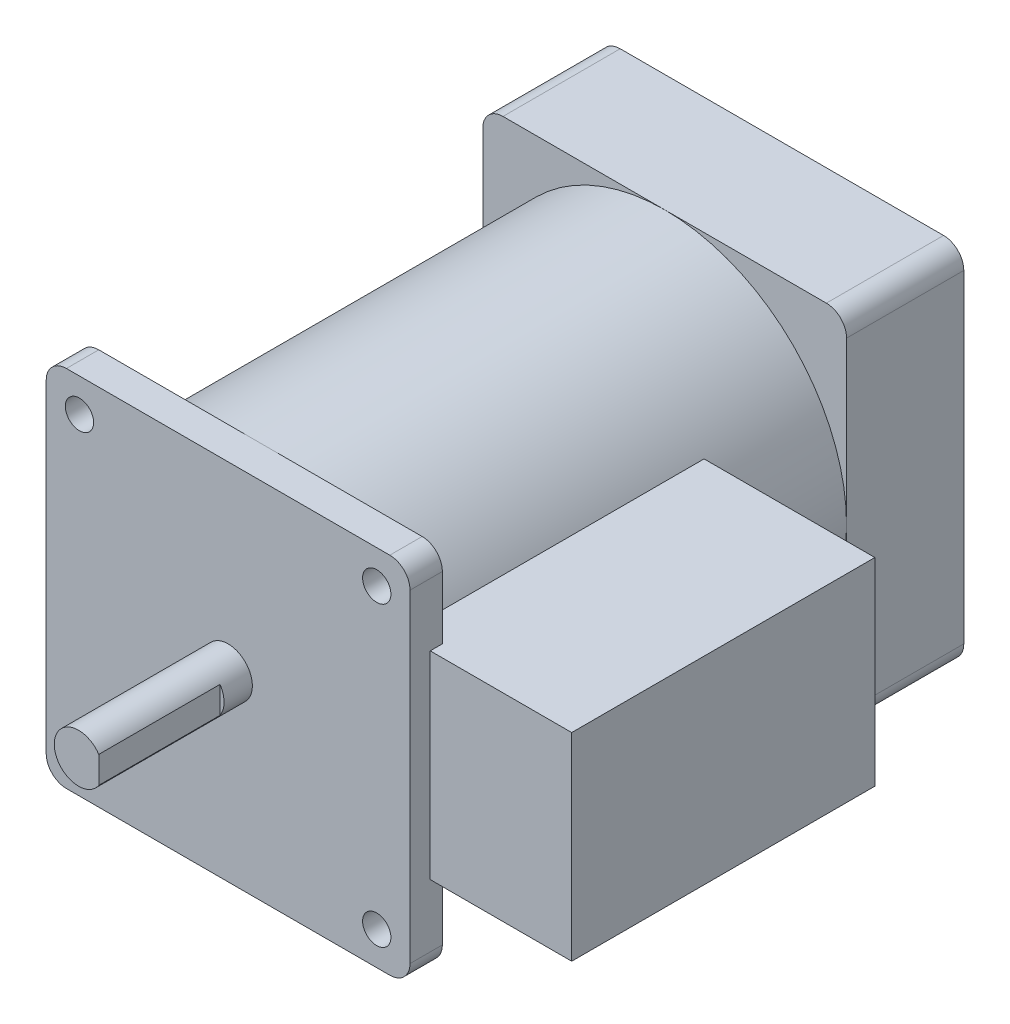
from build123d import *

# Parameters (mm, degrees)
SKETCH_1_W               = 90
SKETCH_1_H               = 90
EXTRUDE_1_DEPTH          = 8
SKETCH_2_R               = 45
EXTRUDE_2_DEPTH          = 100
SKETCH_3_W               = 90
SKETCH_3_H               = 90
EXTRUDE_3_DEPTH          = 29
SKETCH_4_R               = 6
EXTRUDE_4_DEPTH          = 37
SKETCH_6_W               = 75
SKETCH_6_H               = 49
EXTRUDE_5_DEPTH          = 80
SKETCH_7_R               = 3.5
CUT_EXTRUDE_1_DEPTH      = 8
FILLET_1_R               = 5
FILLET_2_R               = 5
SKETCH_9_W               = 30
SKETCH_9_H               = 15.937749453
CUT_EXTRUDE_2_DEPTH      = 1
PATTERN_CIRCULAR_1_COUNT = 4


with BuildPart() as part:
    # 草图1 → 凸台-拉伸1 (new body)
    with BuildSketch(Plane.XY):
        Rectangle(SKETCH_1_W, SKETCH_1_H)
    extrude(amount=EXTRUDE_1_DEPTH)

    # 草图2 → 凸台-拉伸2 (add)
    with BuildSketch(Plane(origin=(0, 0, 0), x_dir=(-1, 0, 0), z_dir=(0, 0, -1))):
        Circle(SKETCH_2_R)
    extrude(amount=EXTRUDE_2_DEPTH)

    # 草图3 → 凸台-拉伸3 (add)
    with BuildSketch(Plane(origin=(0, 0, -100), x_dir=(-1, 0, 0), z_dir=(0, 0, -1))):
        Rectangle(SKETCH_3_W, SKETCH_3_H)
    extrude(amount=EXTRUDE_3_DEPTH)

    # 草图4 → 凸台-拉伸4 (add)
    with BuildSketch(Plane.XY.offset(8)):
        Circle(SKETCH_4_R)
    extrude(amount=EXTRUDE_4_DEPTH)

    # 草图6 → 凸台-拉伸5 (add)
    with BuildSketch(Plane(origin=(0, 0, 0), x_dir=(0, 0, -1), z_dir=(1, 0, 0))):
        with Locations((34.5, 0)):
            Rectangle(SKETCH_6_W, SKETCH_6_H)
    extrude(amount=EXTRUDE_5_DEPTH)

    # 草图7 → 切除-拉伸1 (cut)
    with BuildSketch(Plane.XY.offset(8)):
        with Locations((-36.769552622, 36.769552622)):
            Circle(SKETCH_7_R)
    cut_extrude_1 = extrude(amount=-CUT_EXTRUDE_1_DEPTH, mode=Mode.SUBTRACT)

    # 圆角1
    fillet_1_edges = [part.edges().sort_by_distance(p)[0] for p in [
        (-45, 45, 4),
        (45, 45, 4),
        (45, -45, 4),
        (-45, -45, 4),
    ]]
    fillet(fillet_1_edges, radius=FILLET_1_R)

    # 圆角2
    fillet_2_edges = [part.edges().sort_by_distance(p)[0] for p in [
        (45, 45, -114.5),
        (45, -45, -114.5),
        (-45, -45, -114.5),
        (-45, 45, -114.5),
    ]]
    fillet(fillet_2_edges, radius=FILLET_2_R)

    # 草图9 → 切除-拉伸2 (cut)
    with BuildSketch(Plane(origin=(6, 0, 0), x_dir=(0, 0, -1), z_dir=(1, 0, 0))):
        with Locations((-30, -0.084649365)):
            Rectangle(SKETCH_9_W, SKETCH_9_H)
    extrude(amount=-CUT_EXTRUDE_2_DEPTH, mode=Mode.SUBTRACT)

    # 阵列(圆周)1: 切除-拉伸1 ×4 about axis
    pattern_circular_1_axis = Axis((0, 0, 0), (0, 0, 1))
    for i in range(1, PATTERN_CIRCULAR_1_COUNT):
        add(cut_extrude_1.rotate(pattern_circular_1_axis, i * 360 / PATTERN_CIRCULAR_1_COUNT), mode=Mode.SUBTRACT)


solid = part.part
